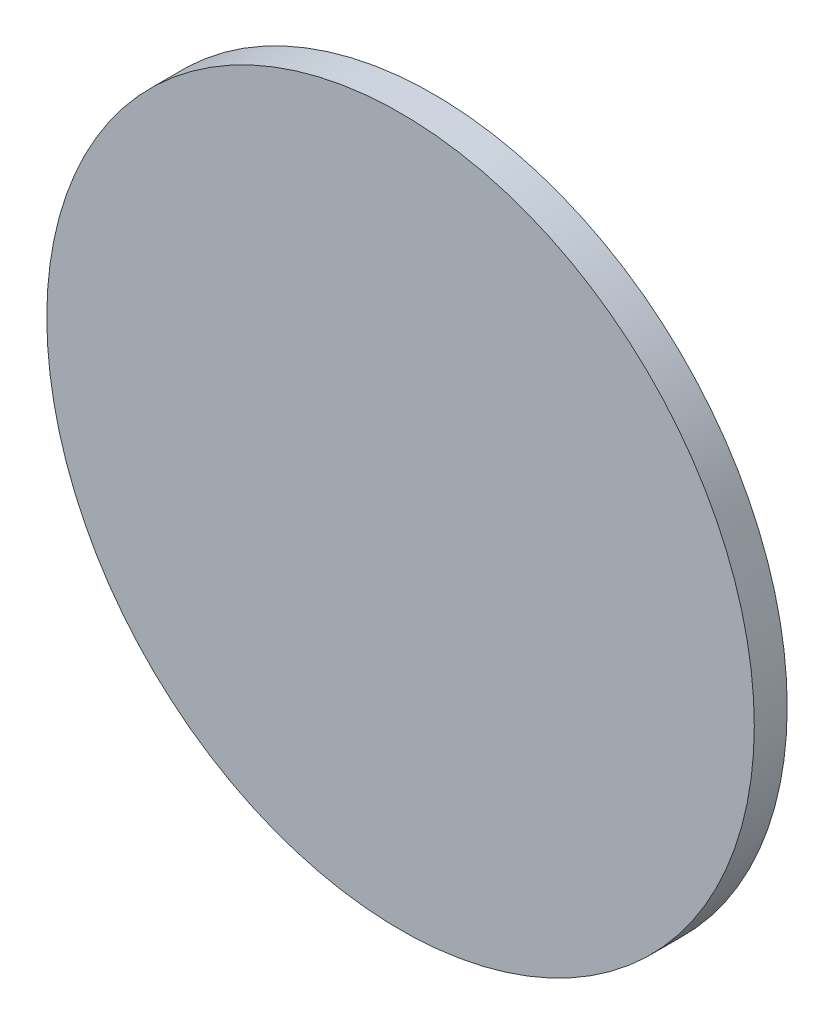
from build123d import *

# Parameters (mm, degrees)
SKETCH1_R           = 215
BOSS_EXTRUDE1_DEPTH = 20


with BuildPart() as part:
    # Sketch1 → Boss-Extrude1 (new body)
    with BuildSketch(Plane.XY):
        Circle(SKETCH1_R)
    extrude(amount=BOSS_EXTRUDE1_DEPTH)


solid = part.part
